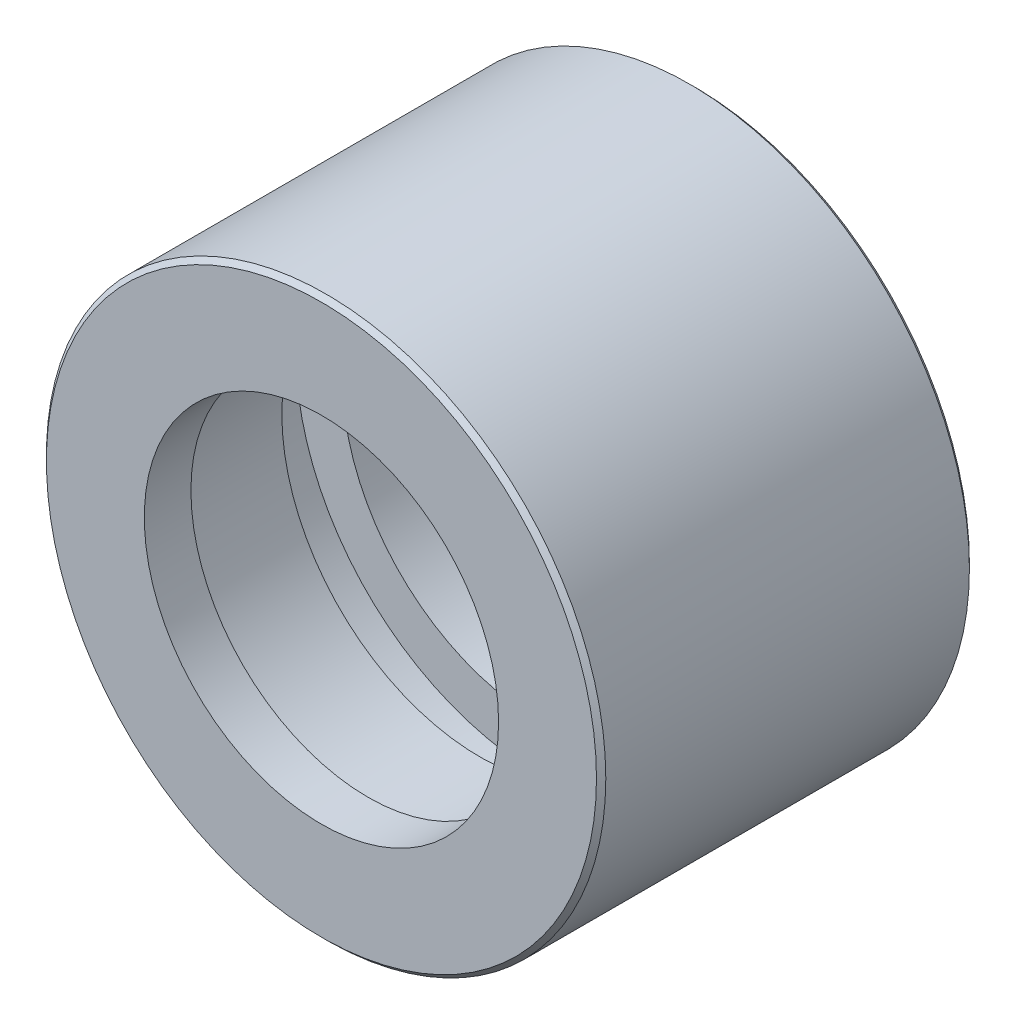
from build123d import *

# Parameters (mm, degrees)
SKETCH_1_R          = 60
EXTRUDE_1_DEPTH     = 80
SKETCH_2_R          = 42.5
CUT_EXTRUDE_1_DEPTH = 70
SKETCH_3_R          = 38
CUT_EXTRUDE_2_DEPTH = 70
CHAMFER_1_SIZE      = 1
SKETCH_4_R          = 52.5
SKETCH_4_R_2        = 42.5
CUT_EXTRUDE_3_DEPTH = 13
SKETCH_5_R          = 52.5
SKETCH_5_R_2        = 42.5
CUT_EXTRUDE_4_DEPTH = 13


with BuildPart() as part:
    # 草图1 → 凸台-拉伸1 (new body)
    with BuildSketch(Plane.XY):
        Circle(SKETCH_1_R)
    extrude(amount=EXTRUDE_1_DEPTH)

    # 草图2 → 切除-拉伸1 (cut)
    with BuildSketch(Plane(origin=(0, 0, 0), x_dir=(-1, 0, 0), z_dir=(0, 0, -1))):
        Circle(SKETCH_2_R)
    extrude(amount=-CUT_EXTRUDE_1_DEPTH, mode=Mode.SUBTRACT)

    # 草图3 → 切除-拉伸2 (cut)
    with BuildSketch(Plane.XY.offset(80)):
        Circle(SKETCH_3_R)
    extrude(amount=-CUT_EXTRUDE_2_DEPTH, mode=Mode.SUBTRACT)

    # 倒角1
    chamfer_1_edges = [part.edges().sort_by_distance(p)[0] for p in [
        (-60, 0, 0),
        (-60, 0, 80),
    ]]
    chamfer(chamfer_1_edges, length=CHAMFER_1_SIZE)

    # 草图4 → 切除-拉伸3 (cut)
    with BuildSketch(Plane(origin=(0, 0, 10), x_dir=(-1, 0, 0), z_dir=(0, 0, -1))):
        Circle(SKETCH_4_R)
        Circle(SKETCH_4_R_2, mode=Mode.SUBTRACT)
    extrude(amount=-CUT_EXTRUDE_3_DEPTH, mode=Mode.SUBTRACT)

    # 草图5 → 切除-拉伸4 (cut)
    with BuildSketch(Plane(origin=(0, 0, 33), x_dir=(-1, 0, 0), z_dir=(0, 0, -1))):
        Circle(SKETCH_5_R)
        Circle(SKETCH_5_R_2, mode=Mode.SUBTRACT)
    extrude(amount=-CUT_EXTRUDE_4_DEPTH, mode=Mode.SUBTRACT)


solid = part.part
